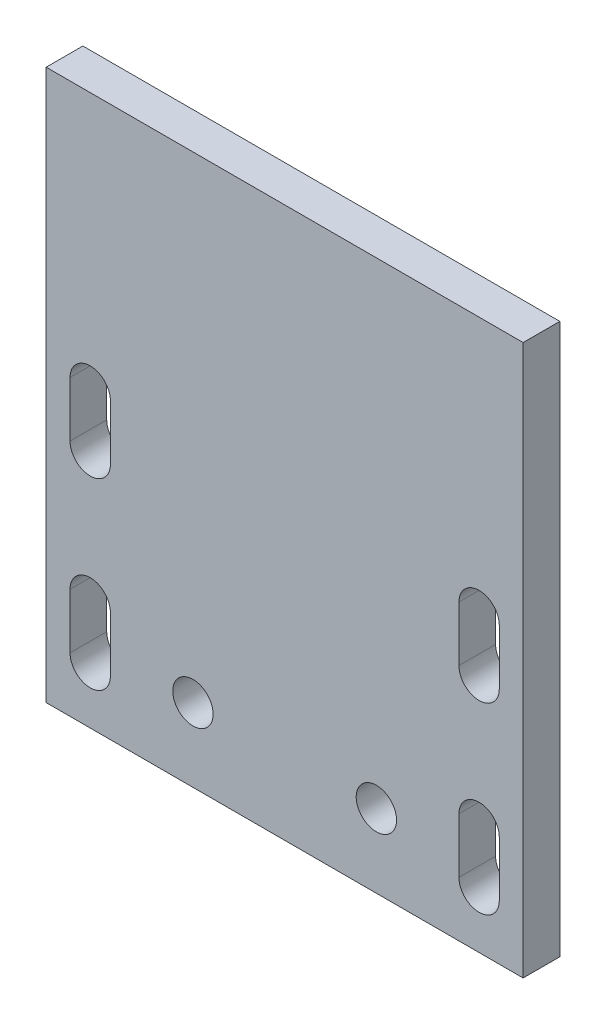
SolidWorks part; units mm, degrees
material "普通碳钢"
ref_plane "Front Plane" through (0, 0, 0) normal (0, 0, 1) x (1, 0, 0)
ref_plane "Top Plane" through (0, 0, 0) normal (0, 1, 0) x (1, 0, 0)
ref_plane "Right Plane" through (0, 0, 0) normal (1, 0, 0) x (0, 0, -1)
sketch "Sketch1" plane through (0, 0, 0) normal (0, 0, 1) x (1, 0, 0)
  line L1 (0, 0) -> (130, 0)
  line L2 (0, 0) -> (0, 130)
  line L3 (0, 130) -> (130, 130)
  line L4 (130, 0) -> (130, 130)
  dimension "D1" = 130
  dimension "D2" = 130
extrude "Boss-Extrude1" add sketch "Sketch1" along normal blind 10
hole_wizard "Ø11.0 (11) Diameter Hole1" positions "Sketch2" profile "Sketch3" hole size "Ø11.0" standard "GB" end condition through all
sketch "Sketch2" plane through (0, 0, 10) normal (0, 0, 1) x (1, 0, 0)
  line L0 (40, 20) -> (90, 20) construction
  line L2 (65, 20) -> (65, 0) construction
  line L3 (0, 0) -> (130, 0) construction
  point P0 (40, 20)
  point P2 (90, 20)
  dimension "D1" = 20
  dimension "D2" = 50
sketch "Sketch3" plane through (40, 20, 10) normal (1, 0, 0) x (0, -1, 0)
  line L0 (0, 0) -> (0, 10)
  line L1 (0, 10) -> (5.5, 10)
  line L2 (5.5, 10) -> (5.5, 0)
  line L5 (5.5, 0) -> (0, 0)
  line L11 (0, -6.35) -> (0, 107.95) construction
  dimension "通孔孔直径" = 11
  dimension "通孔孔深度" = 10
sketch "Sketch4" plane through (0, 130, 0) normal (0, 1, 0) x (1, 0, 0)
  line L4 (130, 0) -> (0, 0)
  line L5 (0, 0) -> (0, -10)
  line L6 (0, -10) -> (130, -10)
  line L7 (130, -10) -> (130, 0)
  line L8 (130, 0) -> (0, 0)
  line L9 (0, 0) -> (0, -10)
  line L10 (0, -10) -> (130, -10)
  line L11 (130, -10) -> (130, 0)
  dimension "D1" = 0
extrude "Boss-Extrude2" add sketch "Sketch4" along normal blind 20
hole_wizard "M6 Clearance Hole1" positions "Sketch5" profile "Sketch6" hole size "M6" standard "GB" end condition through all
sketch "Sketch5" plane through (0, 0, 0) normal (0, 0, -1) x (-1, 0, 0)
  line L0 (0, 0) -> (-130, 0) construction
  line L1 (0, 150) -> (0, 0) construction
  line L2 (-130, 0) -> (-130, 150) construction
  point P0 (-118, 68.5)
  point P2 (-118, 18.5)
  point P4 (-12, 68.5)
  point P6 (-12, 18.5)
  dimension "D1" = 50
  dimension "D2" = 18.5
  dimension "D3" = 12
  dimension "D4" = 12
sketch "Sketch6" plane through (118, 68.5, 0) normal (1, 0, 0) x (0, 1, 0)
  line L0 (0, 0) -> (0, 10)
  line L1 (0, 10) -> (3.5, 10)
  line L2 (3.5, 10) -> (3.5, 0)
  line L5 (3.5, 0) -> (0, 0)
  line L11 (0, -6.35) -> (0, 107.95) construction
  dimension "通孔孔直径" = 7
  dimension "通孔孔深度" = 10
sketch "Sketch8" plane through (0, 0, 0) normal (0, 0, -1) x (-1, 0, 0)
  line L0 (-118, 15) -> (-118, 30) construction
  line L3 (-123.5, 15) -> (-123.5, 30)
  line L4 (-112.5, 15) -> (-112.5, 30)
  line L5 (-118, 65) -> (-118, 80) construction
  line L6 (-123.5, 65) -> (-123.5, 80)
  line L7 (-112.5, 65) -> (-112.5, 80)
  line L8 (-12, 65) -> (-12, 80) construction
  line L9 (-17.5, 65) -> (-17.5, 80)
  line L10 (-6.5, 65) -> (-6.5, 80)
  line L11 (-12, 15) -> (-12, 30) construction
  line L12 (-17.5, 15) -> (-17.5, 30)
  line L13 (-6.5, 15) -> (-6.5, 30)
  circle A3 centre (-118, 18.5) radius 3.5 construction
  arc A4 (-123.5, 15) -> (-112.5, 15) centre (-118, 15) ccw
  arc A5 (-112.5, 30) -> (-123.5, 30) centre (-118, 30) ccw
  circle A6 centre (-118, 68.5) radius 3.5 construction
  arc A7 (-123.5, 65) -> (-112.5, 65) centre (-118, 65) ccw
  arc A8 (-112.5, 80) -> (-123.5, 80) centre (-118, 80) ccw
  circle A9 centre (-12, 68.5) radius 3.5 construction
  arc A10 (-17.5, 65) -> (-6.5, 65) centre (-12, 65) ccw
  arc A11 (-6.5, 80) -> (-17.5, 80) centre (-12, 80) ccw
  circle A12 centre (-12, 18.5) radius 3.5 construction
  arc A13 (-17.5, 15) -> (-6.5, 15) centre (-12, 15) ccw
  arc A14 (-6.5, 30) -> (-17.5, 30) centre (-12, 30) ccw
  point P5 (-118, 22.5)
  point P10 (-118, 72.5)
  point P21 (-12, 72.5)
  point P31 (-12, 22.5)
  dimension "D1" = 11
  dimension "D2" = 15
extrude "Cut-Extrude1" cut sketch "Sketch8" against normal through all
